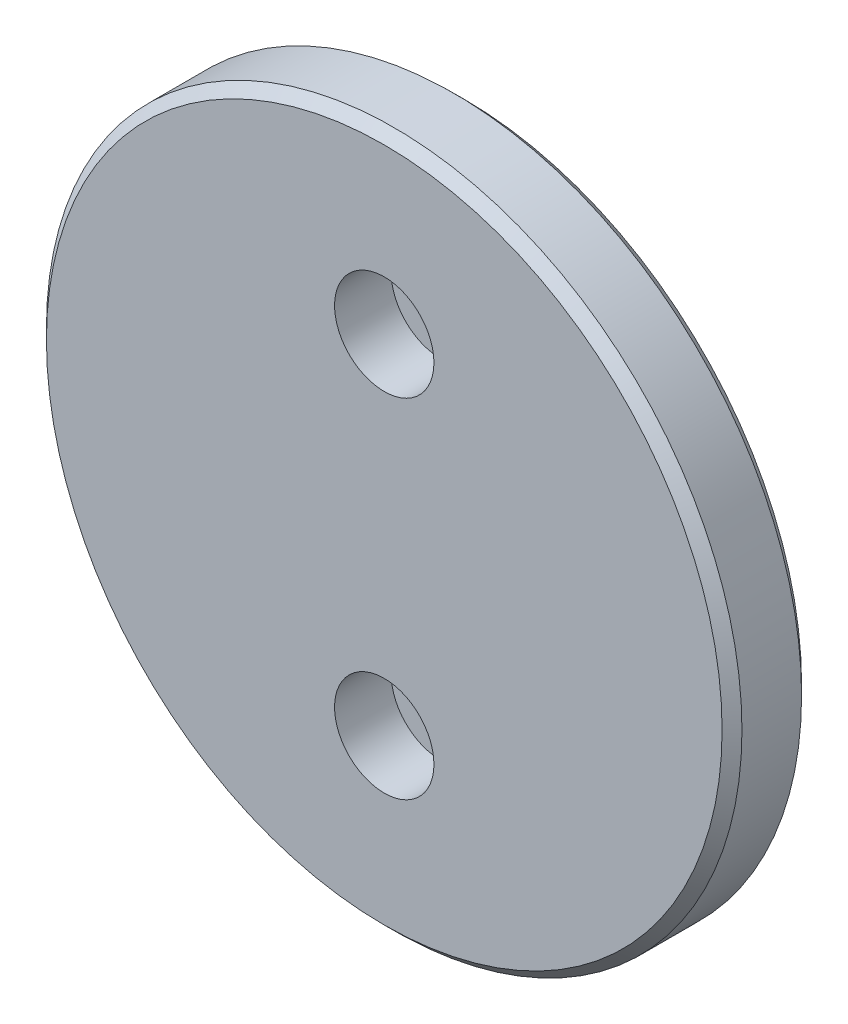
SolidWorks part; units mm, degrees
material "Q235-A"
ref_plane "前视基准面" through (0, 0, 0) normal (0, 0, 1) x (1, 0, 0)
ref_plane "上视基准面" through (0, 0, 0) normal (0, 1, 0) x (1, 0, 0)
ref_plane "右视基准面" through (0, 0, 0) normal (1, 0, 0) x (0, 0, -1)
sketch "草图1" plane through (0, 0, 0) normal (0, 0, 1) x (1, 0, 0)
  circle A0 centre (0, 0) radius 35
  dimension "D1" = 70
extrude "凸台-拉伸1" add sketch "草图1" along normal blind 8
hole_wizard "打孔尺寸根据内六角圆柱头螺钉的类型1" positions "草图3" profile "草图2" counterbore size "M5" standard "Gb" end condition through all
sketch "草图3" plane through (0, 0, 8) normal (0, 0, 1) x (1, 0, 0)
  line L0 (0, 0) -> (0, 30) construction
  line L4 (0, 0) -> (40, 0) construction
  point P0 (0, 17.5)
  point P2 (0, -17.5)
  dimension "D1" = 35
sketch "草图2" plane through (0, 17.5, 8) normal (1, 0, 0) x (0, -1, 0)
  line L0 (0, 0) -> (0, 8)
  line L1 (0, 8) -> (2.75, 8)
  line L3 (2.75, 8) -> (2.75, 5.7)
  line L4 (2.75, 5.7) -> (5, 5.7)
  line L5 (5, 5.7) -> (5, 0)
  line L7 (5, 0) -> (0, 0)
  line L11 (0, -6.35) -> (0, 107.95) construction
  dimension "通孔孔直径" = 5.5
  dimension "通孔孔深度" = 8
  dimension "柱形沉头孔直径" = 10
  dimension "柱形沉头孔深度" = 5.7
chamfer "倒角1" distance 1 angle 45 2 edges at (35, 0, 0) (35, 0, 8)
